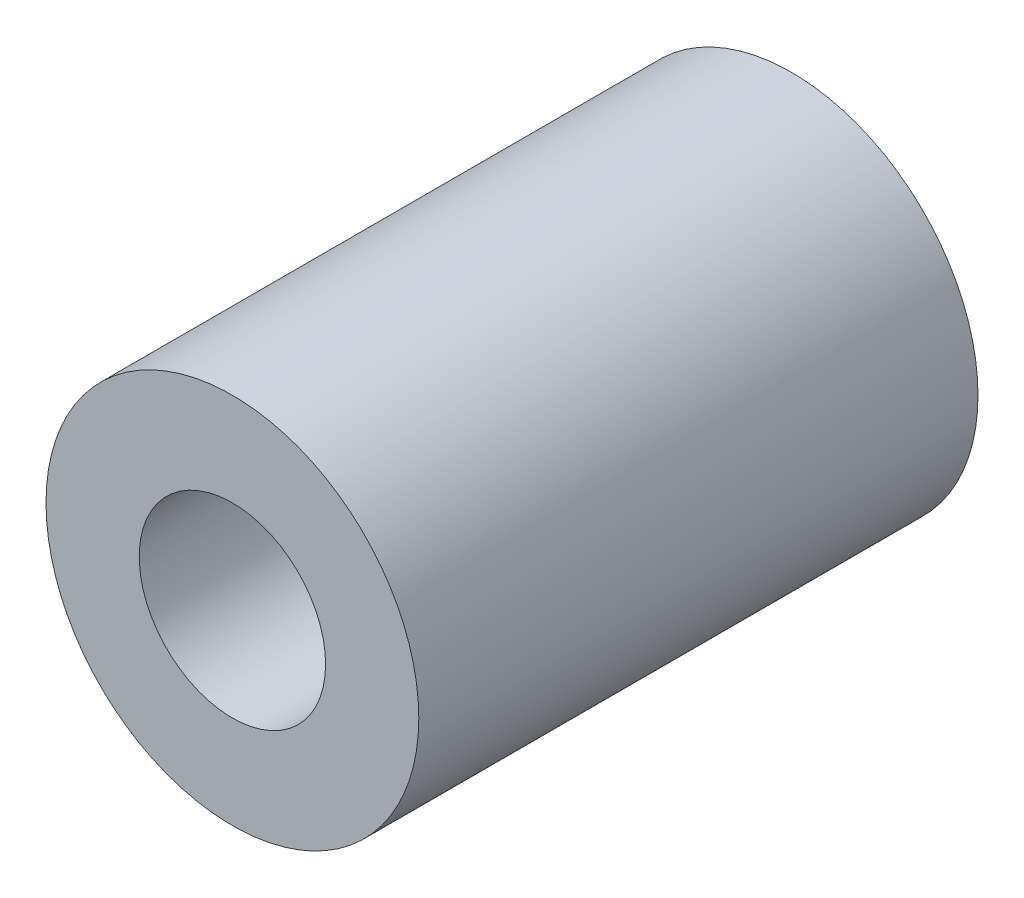
SolidWorks part; units mm, degrees
ref_plane "前视基准面" through (0, 0, 0) normal (0, 0, 1) x (1, 0, 0)
ref_plane "上视基准面" through (0, 0, 0) normal (0, 1, 0) x (1, 0, 0)
ref_plane "右视基准面" through (0, 0, 0) normal (1, 0, 0) x (0, 0, -1)
other "Configuration Table"
sketch "草图1" plane through (0, 0, 0) normal (0, 0, 1) x (1, 0, 0)
  circle A0 centre (0, 0) radius 8
  circle A1 centre (0, 0) radius 4
  point P0 (0, 0)
  dimension "D1" = 8
  dimension "D2" = 16
extrude "凸台-拉伸1" add sketch "草图1" against normal mid plane 24
